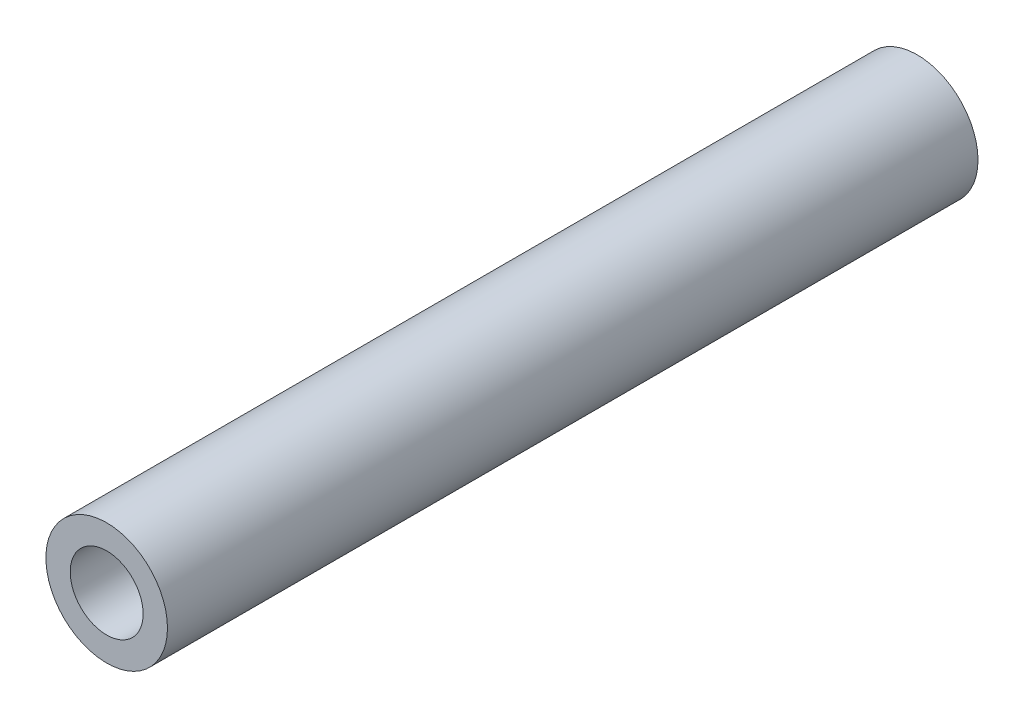
from build123d import *

# Parameters (mm, degrees)
SKETCH_1_R      = 1.5
SKETCH_1_R_2    = 0.9
EXTRUDE_1_DEPTH = 20


with BuildPart() as part:
    # 草图1 → 拉伸1 (new body)
    with BuildSketch(Plane.XY):
        Circle(SKETCH_1_R)
        Circle(SKETCH_1_R_2, mode=Mode.SUBTRACT)
    extrude(amount=EXTRUDE_1_DEPTH)


solid = part.part
